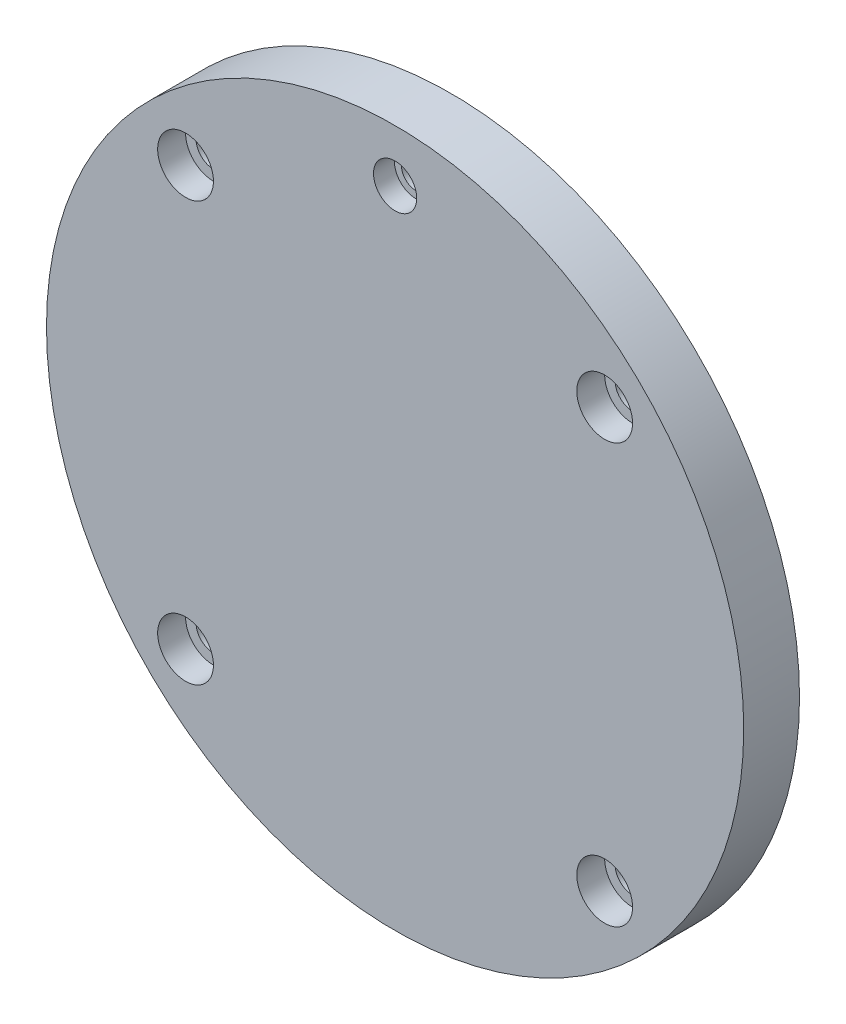
from build123d import *

# Parameters (mm, degrees)
SKETCH1_R           = 50
BOSS_EXTRUDE1_DEPTH = 8
SKETCH2_R           = 4
CUT_EXTRUDE1_DEPTH  = 4
SKETCH3_R           = 3.1
CUT_EXTRUDE2_DEPTH  = 3
SKETCH4_R           = 2.5
SKETCH4_R_2         = 2.1
CUT_EXTRUDE3_DEPTH  = 71.823724839
SKETCH5_R           = 2.1
CUT_EXTRUDE4_DEPTH  = 5


with BuildPart() as part:
    # Sketch1 → Boss-Extrude1 (new body)
    with BuildSketch(Plane.XY):
        Circle(SKETCH1_R)
    extrude(amount=BOSS_EXTRUDE1_DEPTH)

    # Sketch2 → Cut-Extrude1 (cut)
    with BuildSketch(Plane.XY.offset(8)):
        with Locations((-30.054076263, 30.05)):
            Circle(SKETCH2_R)
        with Locations((30.054076263, 30.05)):
            Circle(SKETCH2_R)
        with Locations((-30.054076263, -30.05)):
            Circle(SKETCH2_R)
        with Locations((30.054076263, -30.05)):
            Circle(SKETCH2_R)
    extrude(amount=-CUT_EXTRUDE1_DEPTH, mode=Mode.SUBTRACT)

    # Sketch3 → Cut-Extrude2 (cut)
    with BuildSketch(Plane.XY.offset(8)):
        with Locations((0, 42.5)):
            Circle(SKETCH3_R)
    extrude(amount=-CUT_EXTRUDE2_DEPTH, mode=Mode.SUBTRACT)

    # Sketch4 → Cut-Extrude3 (cut, through all)
    with BuildSketch(Plane.XY.offset(4)):
        with Locations((-30.054076263, 30.05)):
            Circle(SKETCH4_R)
        with Locations((30.054076263, 30.05)):
            Circle(SKETCH4_R)
        with Locations((-30.054076263, -30.05)):
            Circle(SKETCH4_R)
        with Locations((30.054076263, -30.05)):
            Circle(SKETCH4_R)
        with Locations((0, 42.5)):
            Circle(SKETCH4_R_2)
    extrude(amount=-CUT_EXTRUDE3_DEPTH, mode=Mode.SUBTRACT)

    # Sketch5 → Cut-Extrude4 (cut)
    with BuildSketch(Plane.XY.offset(5)):
        with Locations((0, 42.5)):
            Circle(SKETCH5_R)
    extrude(amount=-CUT_EXTRUDE4_DEPTH, mode=Mode.SUBTRACT)


solid = part.part
